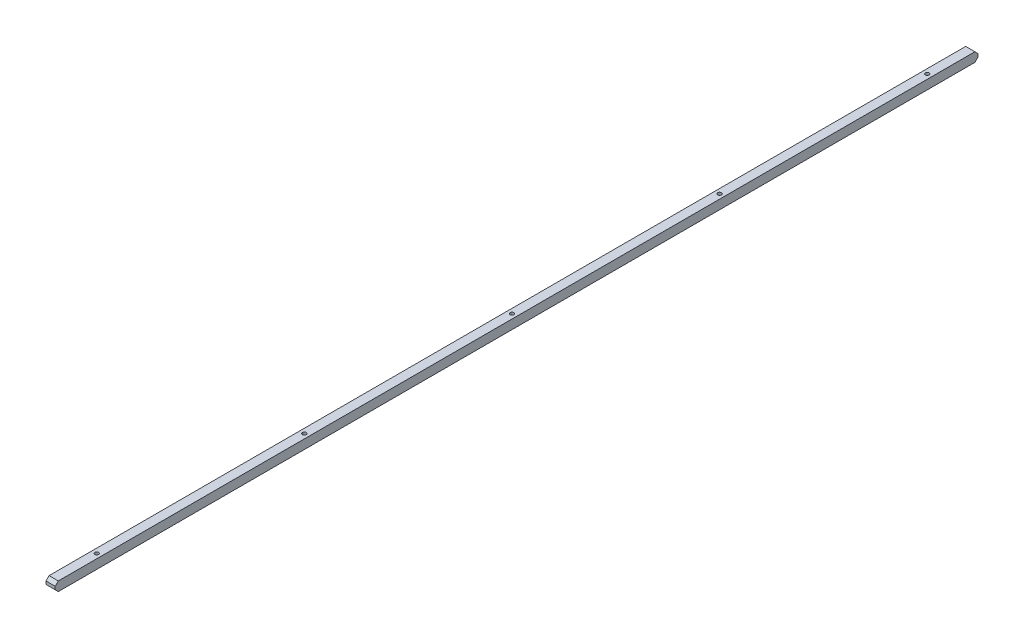
from build123d import *

# Parameters (mm, degrees)
SKETCH_1_W         = 6
SKETCH_1_H         = 6
EXTRUDE_1_DEPTH    = 600
HOLE_WIZARD_M3_1_D = 2.5
CHAMFER_1_SIZE     = 2


with BuildPart() as part:
    # 草图1 → 凸台-拉伸1 (new body)
    with BuildSketch(Plane.XY):
        Rectangle(SKETCH_1_W, SKETCH_1_H)
    extrude(amount=EXTRUDE_1_DEPTH)

    # M3 螺纹孔1 (through all)
    with Locations(Plane(origin=(0, 3, 165), x_dir=(0, 0, 1), z_dir=(0, 1, 0))):
        with Locations((0, 0), (135, 0), (270, 0), (405, 0), (-135, 0)):
            Hole(HOLE_WIZARD_M3_1_D / 2)

    # 倒角1
    chamfer_1_edges = [part.edges().sort_by_distance(p)[0] for p in [
        (0, -3, 600),
        (0, -3, 0),
        (0, 3, 0),
        (0, 3, 600),
    ]]
    chamfer(chamfer_1_edges, length=CHAMFER_1_SIZE)


solid = part.part
